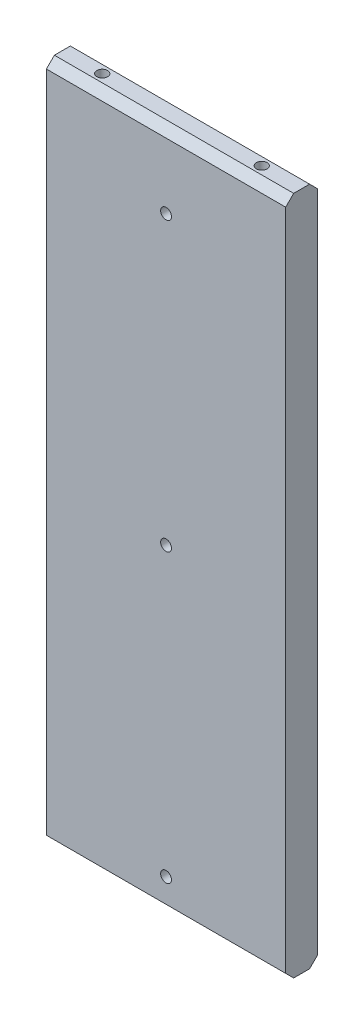
from build123d import *

# Parameters (mm, degrees)
SKETCH1_W             = 150
SKETCH1_H             = 426
BOSS_EXTRUDE1_DEPTH   = 20
SKETCH2_W             = 20
SKETCH2_H             = 400
CUT_EXTRUDE1_DEPTH    = 3
M8_TAPPED_HOLE2_D     = 6.8
M8_TAPPED_HOLE2_DEPTH = 19.75
M8_TAPPED_HOLE2_TIP   = 2.042926105
M8_TAPPED_HOLE1_D     = 6.8
M8_TAPPED_HOLE1_DEPTH = 20
M8_TAPPED_HOLE1_TIP   = 2.042926105
CHAMFER1_SIZE         = 5
CHAMFER2_SIZE         = 5


with BuildPart() as part:
    # Sketch1 → Boss-Extrude1 (new body)
    with BuildSketch(Plane.XY):
        with Locations((75, 213)):
            Rectangle(SKETCH1_W, SKETCH1_H)
    extrude(amount=BOSS_EXTRUDE1_DEPTH)

    # Sketch2 → Cut-Extrude1 (cut)
    with BuildSketch(Plane(origin=(0, 0, 0), x_dir=(-1, 0, 0), z_dir=(0, 0, -1))):
        with Locations((-75, 200)):
            Rectangle(SKETCH2_W, SKETCH2_H)
    extrude(amount=-CUT_EXTRUDE1_DEPTH, mode=Mode.SUBTRACT)

    # M8 Tapped Hole2
    with Locations(Plane(origin=(0, 0, 3), x_dir=(-1, 0, 0), z_dir=(0, 0, -1))):
        with Locations((-75, 20), (-75, 200), (-75, 380)):
            Hole(M8_TAPPED_HOLE2_D / 2, depth=M8_TAPPED_HOLE2_DEPTH)
            with Locations((0, 0, -(M8_TAPPED_HOLE2_DEPTH + M8_TAPPED_HOLE2_TIP / 2))):  # 118° drill point
                Cone(0, M8_TAPPED_HOLE2_D / 2, M8_TAPPED_HOLE2_TIP, mode=Mode.SUBTRACT)

    # M8 Tapped Hole1
    with Locations(Plane(origin=(0, 426, 0), x_dir=(1, 0, 0), z_dir=(0, 1, 0))):
        with Locations((25, -10), (125, -10)):
            Hole(M8_TAPPED_HOLE1_D / 2, depth=M8_TAPPED_HOLE1_DEPTH)
            with Locations((0, 0, -(M8_TAPPED_HOLE1_DEPTH + M8_TAPPED_HOLE1_TIP / 2))):  # 118° drill point
                Cone(0, M8_TAPPED_HOLE1_D / 2, M8_TAPPED_HOLE1_TIP, mode=Mode.SUBTRACT)

    # Chamfer1
    chamfer1_edges = [part.edges().sort_by_distance(p)[0] for p in [
        (75, 0, 20),
        (32.5, 0, 0),
    ]]
    chamfer(chamfer1_edges, length=CHAMFER1_SIZE)

    # Chamfer2
    chamfer2_edges = [part.edges().sort_by_distance(p)[0] for p in [
        (75, 426, 20),
        (75, 426, 0),
    ]]
    chamfer(chamfer2_edges, length=CHAMFER2_SIZE)


solid = part.part
